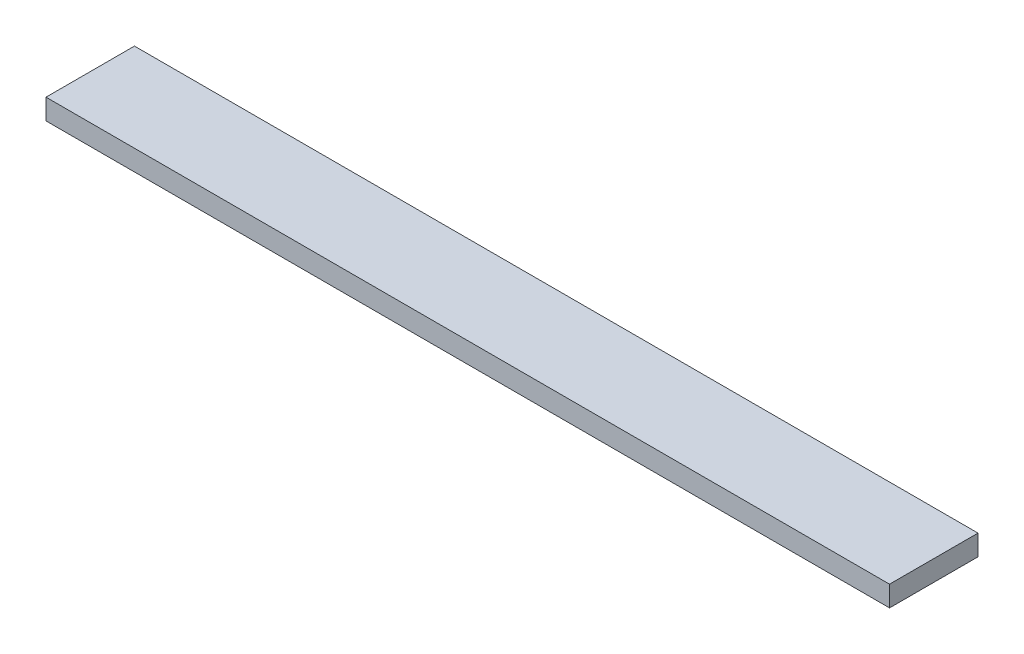
from build123d import *

# Parameters (mm, degrees)
SKETCH1_W           = 41
SKETCH1_H           = 4.3
BOSS_EXTRUDE1_DEPTH = 1


with BuildPart() as part:
    # Sketch1 → Boss-Extrude1 (new body)
    with BuildSketch(Plane(origin=(0, 0, 0), x_dir=(1, 0, 0), z_dir=(0, 1, 0))):
        with Locations((20.5, 0)):
            Rectangle(SKETCH1_W, SKETCH1_H)
    extrude(amount=BOSS_EXTRUDE1_DEPTH)


solid = part.part
